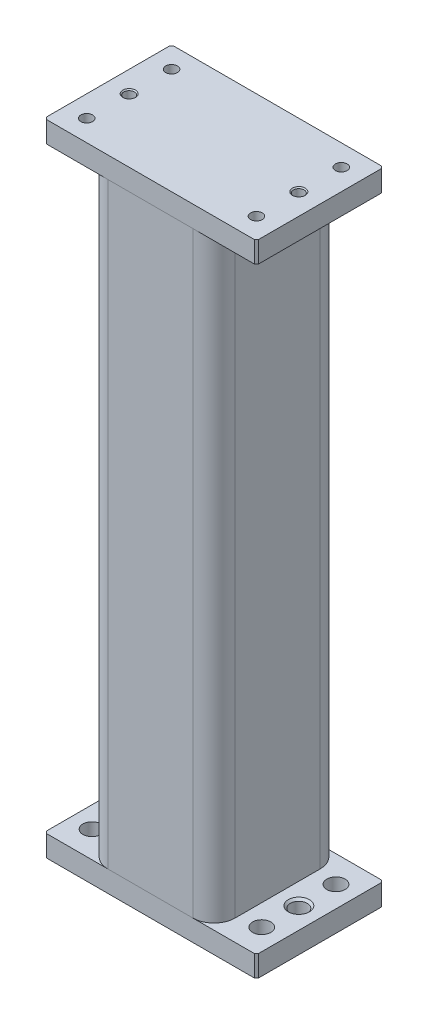
from build123d import *

# Parameters (mm, degrees)
MEMBER_1_DEPTH                   = 281.5
SKETCH_2_W                       = 100
SKETCH_2_H                       = 60
EXTRUDE_1_DEPTH                  = 10
SKETCH_3_W                       = 100
SKETCH_3_H                       = 60
EXTRUDE_2_DEPTH                  = 10
HOLE_WIZARD_8_6_8_6_1_AT_2_COUNT = 2
HOLE_WIZARD_8_6_8_6_1_AT_2_PITCH = 35
HOLE_WIZARD_8_6_8_6_1_AT_3_COUNT = 2
HOLE_WIZARD_8_6_8_6_1_AT_3_PITCH = 80
HOLE_WIZARD_8_6_8_6_1_AT_4_COUNT = 2
HOLE_WIZARD_8_6_8_6_1_AT_4_PITCH = 87.321245983
SKETCH_6_R                       = 4
CUT_EXTRUDE_1_DEPTH              = 298.274704608
CHAMFER_3_SIZE                   = 1
HOLE_WIZARD_5_5_5_5_1_AT_2_COUNT = 2
HOLE_WIZARD_5_5_5_5_1_AT_2_PITCH = 40
HOLE_WIZARD_5_5_5_5_1_AT_3_COUNT = 2
HOLE_WIZARD_5_5_5_5_1_AT_3_PITCH = 80
HOLE_WIZARD_5_5_5_5_1_AT_4_COUNT = 2
HOLE_WIZARD_5_5_5_5_1_AT_4_PITCH = 89.4427191
SKETCH_9_R                       = 2.5
CUT_EXTRUDE_2_DEPTH              = 298.274704608
CHAMFER_4_SIZE                   = 0.5
CHAMFER_5_SIZE                   = 1
CHAMFER_6_SIZE                   = 1


with BuildPart() as part:
    # Sketch11 → Member 1 (new body)
    with BuildSketch(Plane(origin=(0, 0, 0), x_dir=(1, 0, 0), z_dir=(0, 1, 0))):
        with BuildLine():
            Line((-20, -30), (20, -30))
            ThreePointArc((20, -30), (27.071067812, -27.071067812), (30, -20))
            Line((30, -20), (30, 20))
            ThreePointArc((30, 20), (27.071067812, 27.071067812), (20, 30))
            Line((20, 30), (-20, 30))
            ThreePointArc((-20, 30), (-27.071067812, 27.071067812), (-30, 20))
            Line((-30, 20), (-30, -20))
            ThreePointArc((-30, -20), (-27.071067812, -27.071067812), (-20, -30))
        make_face()
        with BuildLine():
            Line((-20, -25), (20, -25))
            ThreePointArc((20, -25), (23.535533906, -23.535533906), (25, -20))
            Line((25, -20), (25, 20))
            ThreePointArc((25, 20), (23.535533906, 23.535533906), (20, 25))
            Line((20, 25), (-20, 25))
            ThreePointArc((-20, 25), (-23.535533906, 23.535533906), (-25, 20))
            Line((-25, 20), (-25, -20))
            ThreePointArc((-25, -20), (-23.535533906, -23.535533906), (-20, -25))
        make_face(mode=Mode.SUBTRACT)
    extrude(amount=MEMBER_1_DEPTH)


with BuildPart() as body_2:
    # 草图2 → 凸台-拉伸1 (new body)
    with BuildSketch(Plane(origin=(0, 281.5, 0), x_dir=(1, 0, 0), z_dir=(0, 1, 0))):
        Rectangle(SKETCH_2_W, SKETCH_2_H)
    extrude(amount=EXTRUDE_1_DEPTH)

    # 草图7 → Ø5.5 (5.5) 直径孔1 (revolve, cut)
    with BuildSketch(Plane(origin=(-40, 281.5, -20), x_dir=(0, 0, -1), z_dir=(1, 0, 0))):
        Polygon((0, 0), (0, 17.19771324), (2.75, 15.61), (2.75, 0), align=None)
    hole_wizard_5_5_5_5_1 = revolve(axis=Axis((-40, 275.15, -20), (0, 1, 0)), mode=Mode.SUBTRACT)

    # Ø5.5 (5.5) 直径孔1 at 2: Ø5.5 (5.5) 直径孔1 ×2
    with Locations(*[(0, 0, i * HOLE_WIZARD_5_5_5_5_1_AT_2_PITCH) for i in range(1, HOLE_WIZARD_5_5_5_5_1_AT_2_COUNT)]):
        add(hole_wizard_5_5_5_5_1, mode=Mode.SUBTRACT)

    # Ø5.5 (5.5) 直径孔1 at 3: Ø5.5 (5.5) 直径孔1 ×2
    with Locations(*[(i * HOLE_WIZARD_5_5_5_5_1_AT_3_PITCH, 0, 0) for i in range(1, HOLE_WIZARD_5_5_5_5_1_AT_3_COUNT)]):
        add(hole_wizard_5_5_5_5_1, mode=Mode.SUBTRACT)

    # Ø5.5 (5.5) 直径孔1 at 4: Ø5.5 (5.5) 直径孔1 ×2
    with Locations(*[Vector(0.894427190999916, 0, 0.447213595499958) * (i * HOLE_WIZARD_5_5_5_5_1_AT_4_PITCH) for i in range(1, HOLE_WIZARD_5_5_5_5_1_AT_4_COUNT)]):
        add(hole_wizard_5_5_5_5_1, mode=Mode.SUBTRACT)

    # 草图9 → 切除-拉伸2 (cut, through all)
    with BuildSketch(Plane.XZ.offset(-281.5)):
        with Locations(Location((40, 0, 0), (0, 0, 270))):
            Circle(SKETCH_9_R)
        with Locations(Location((-40, 0, 0), (0, 0, 270))):
            Circle(SKETCH_9_R)
    extrude(amount=-CUT_EXTRUDE_2_DEPTH, mode=Mode.SUBTRACT)

    # 倒角4
    chamfer_4_edges = [body_2.edges().sort_by_distance(p)[0] for p in [
        (40, 291.5, 2.5),
        (40, 281.5, 2.5),
        (-40, 291.5, 2.5),
        (-40, 281.5, 2.5),
    ]]
    chamfer(chamfer_4_edges, length=CHAMFER_4_SIZE)

    # 倒角6
    chamfer_6_edges = [body_2.edges().sort_by_distance(p)[0] for p in [
        (50, 286.5, 30),
        (-50, 286.5, 30),
        (-50, 286.5, -30),
        (50, 286.5, -30),
    ]]
    chamfer(chamfer_6_edges, length=CHAMFER_6_SIZE)


with BuildPart() as body_3:
    # 草图3 → 凸台-拉伸2 (new body)
    with BuildSketch(Plane.XZ):
        Rectangle(SKETCH_3_W, SKETCH_3_H)
    extrude(amount=EXTRUDE_2_DEPTH)

    # 草图4 → Ø8.6 (8.6) 直径孔1 (revolve, cut)
    with BuildSketch(Plane(origin=(40, 0, -17.5), x_dir=(0, 0, 1), z_dir=(1, 0, 0))):
        Polygon((0, 0), (0, 18.092606158), (4.3, 15.61), (4.3, 0), align=None)
    hole_wizard_8_6_8_6_1 = revolve(axis=Axis((40, 6.35, -17.5), (0, -1, 0)), mode=Mode.SUBTRACT)

    # Ø8.6 (8.6) 直径孔1 at 2: Ø8.6 (8.6) 直径孔1 ×2
    with Locations(*[(0, 0, i * HOLE_WIZARD_8_6_8_6_1_AT_2_PITCH) for i in range(1, HOLE_WIZARD_8_6_8_6_1_AT_2_COUNT)]):
        add(hole_wizard_8_6_8_6_1, mode=Mode.SUBTRACT)

    # Ø8.6 (8.6) 直径孔1 at 3: Ø8.6 (8.6) 直径孔1 ×2
    with Locations(*[(-i * HOLE_WIZARD_8_6_8_6_1_AT_3_PITCH, 0, 0) for i in range(1, HOLE_WIZARD_8_6_8_6_1_AT_3_COUNT)]):
        add(hole_wizard_8_6_8_6_1, mode=Mode.SUBTRACT)

    # Ø8.6 (8.6) 直径孔1 at 4: Ø8.6 (8.6) 直径孔1 ×2
    with Locations(*[Vector(-0.9161573349021891, 0, 0.4008188340197079) * (i * HOLE_WIZARD_8_6_8_6_1_AT_4_PITCH) for i in range(1, HOLE_WIZARD_8_6_8_6_1_AT_4_COUNT)]):
        add(hole_wizard_8_6_8_6_1, mode=Mode.SUBTRACT)

    # 草图6 → 切除-拉伸1 (cut, through all)
    with BuildSketch(Plane(origin=(0, 0, 0), x_dir=(1, 0, 0), z_dir=(0, 1, 0))):
        with Locations(Location((-40, 0, 0), (0, 0, 270))):
            Circle(SKETCH_6_R)
        with Locations(Location((40, 0, 0), (0, 0, 270))):
            Circle(SKETCH_6_R)
    extrude(amount=-CUT_EXTRUDE_1_DEPTH, mode=Mode.SUBTRACT)

    # 倒角3
    chamfer_3_edges = [body_3.edges().sort_by_distance(p)[0] for p in [
        (-40, -10, -4),
        (-40, 0, -4),
        (40, -10, -4),
        (40, 0, -4),
    ]]
    chamfer(chamfer_3_edges, length=CHAMFER_3_SIZE)

    # 倒角5
    chamfer_5_edges = [body_3.edges().sort_by_distance(p)[0] for p in [
        (50, -5, -30),
        (-50, -5, -30),
        (-50, -5, 30),
        (50, -5, 30),
    ]]
    chamfer(chamfer_5_edges, length=CHAMFER_5_SIZE)


solid = Compound([part.part, body_2.part, body_3.part])
